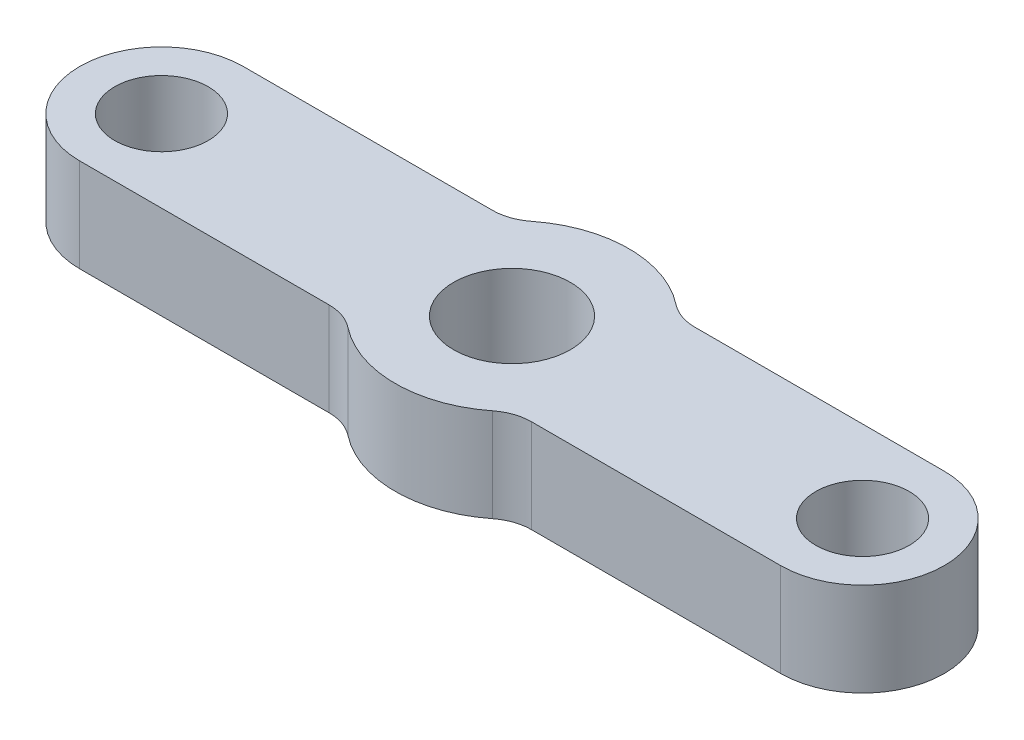
from build123d import *

# Parameters (mm, degrees)
SKETCH1_R           = 5
SKETCH1_R_2         = 4
BOSS_EXTRUDE1_DEPTH = 8
SCALE1_SCALE        = 0.5


with BuildPart() as part:
    # Sketch1 → Boss-Extrude1 (new body)
    with BuildSketch(Plane(origin=(0, 0, 0), x_dir=(1, 0, 0), z_dir=(0, 1, 0))):
        with BuildLine():
            Line((30, 7), (8.660254038, 7))
            ThreePointArc((8.660254038, 7), (7.350946696, 7.22035527), (6.185895741, 7.857142857))
            ThreePointArc((6.185895741, 7.857142857), (0, 10), (-6.185895741, 7.857142857))
            ThreePointArc((-6.185895741, 7.857142857), (-7.350946696, 7.22035527), (-8.660254038, 7))
            Line((-8.660254038, 7), (-30, 7))
            ThreePointArc((-30, 7), (-37, 0), (-30, -7))
            Line((-30, -7), (-8.660254038, -7))
            ThreePointArc((-8.660254038, -7), (-7.350946696, -7.22035527), (-6.185895741, -7.857142857))
            ThreePointArc((-6.185895741, -7.857142857), (0, -10), (6.185895741, -7.857142857))
            ThreePointArc((6.185895741, -7.857142857), (7.350946696, -7.22035527), (8.660254038, -7))
            Line((8.660254038, -7), (30, -7))
            ThreePointArc((30, -7), (37, 0), (30, 7))
        make_face()
        with Locations(Location((0, 0, 0), (0, 0, 270))):
            Circle(SKETCH1_R, mode=Mode.SUBTRACT)
        with Locations(Location((30, 0, 0), (0, 0, 270))):
            Circle(SKETCH1_R_2, mode=Mode.SUBTRACT)
        with Locations(Location((-30, 0, 0), (0, 0, 90))):
            Circle(SKETCH1_R_2, mode=Mode.SUBTRACT)
    extrude(amount=BOSS_EXTRUDE1_DEPTH)


with BuildPart() as part_1:
    # Scale1: scaled about (0, 0, 0)
    add(part.part.scale(SCALE1_SCALE))


solid = part_1.part
